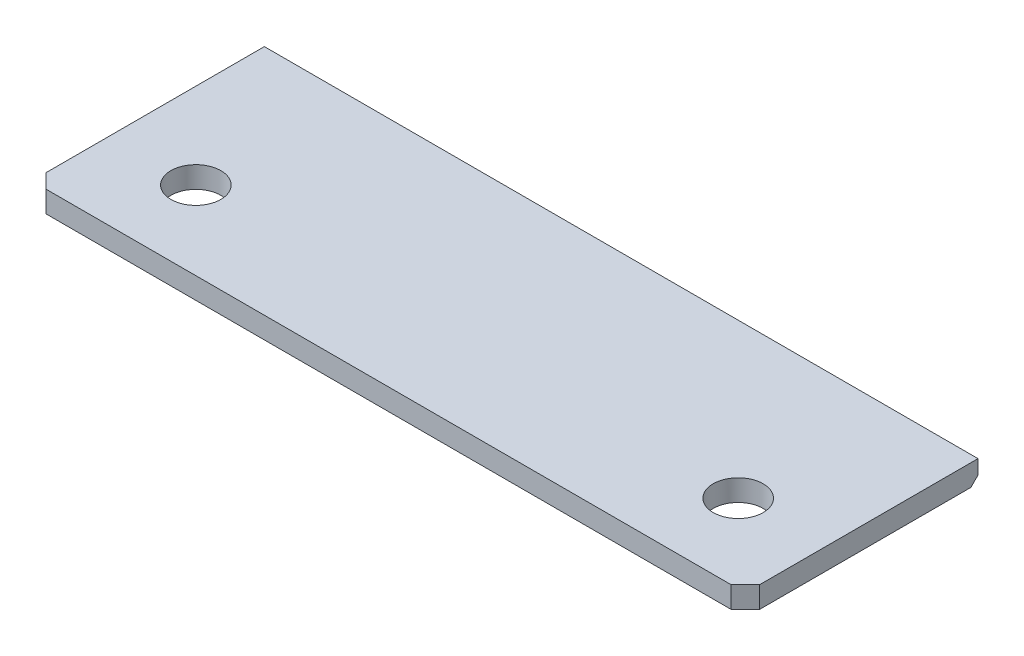
SolidWorks part; units mm, degrees
ref_plane "Front Plane" through (0, 0, 0) normal (0, 0, 1) x (1, 0, 0)
ref_plane "Top Plane" through (0, 0, 0) normal (0, 1, 0) x (1, 0, 0)
ref_plane "Right Plane" through (0, 0, 0) normal (1, 0, 0) x (0, 0, -1)
sketch "Sketch1" plane through (0, 0, 0) normal (0, 1, 0) x (1, 0, 0)
  line L1 (-25, 8.15) -> (25, 8.15)
  line L2 (-25, 8.15) -> (-25, -8.15)
  line L3 (-25, -8.15) -> (25, -8.15)
  line L4 (25, 8.15) -> (25, -8.15)
  line L5 (-25, 8.15) -> (25, -8.15) construction
  line L6 (-25, -8.15) -> (25, 8.15) construction
  point P0 (0, 0)
  dimension "D1" = 16.3
  dimension "D2" = 50
extrude "Boss-Extrude1" add sketch "Sketch1" along normal blind 1.5
sketch "Sketch3" plane through (0, 1.5, 0) normal (0, 1, 0) x (1, 0, 0)
  line L0 (0, 0) -> (0, -50000) construction
  line L1 (-25, -8.15) -> (25, -8.15) construction
  circle A0 centre (-19, -2.65) radius 1.75
  circle A1 centre (19, -2.65) radius 1.75
  dimension "D1" = 3.5
  dimension "D2" = 38
  dimension "D3" = 5.5
extrude "Cut-Extrude2" cut sketch "Sketch3" against normal blind 10
chamfer "Chamfer1" distance 1 angle 45 2 edges at (25, 0.75, 8.15) (-25, 0.75, 8.15)
chamfer "Chamfer2" distance 0.5 angle 45 1 edges at (0, 0, -8.15)
